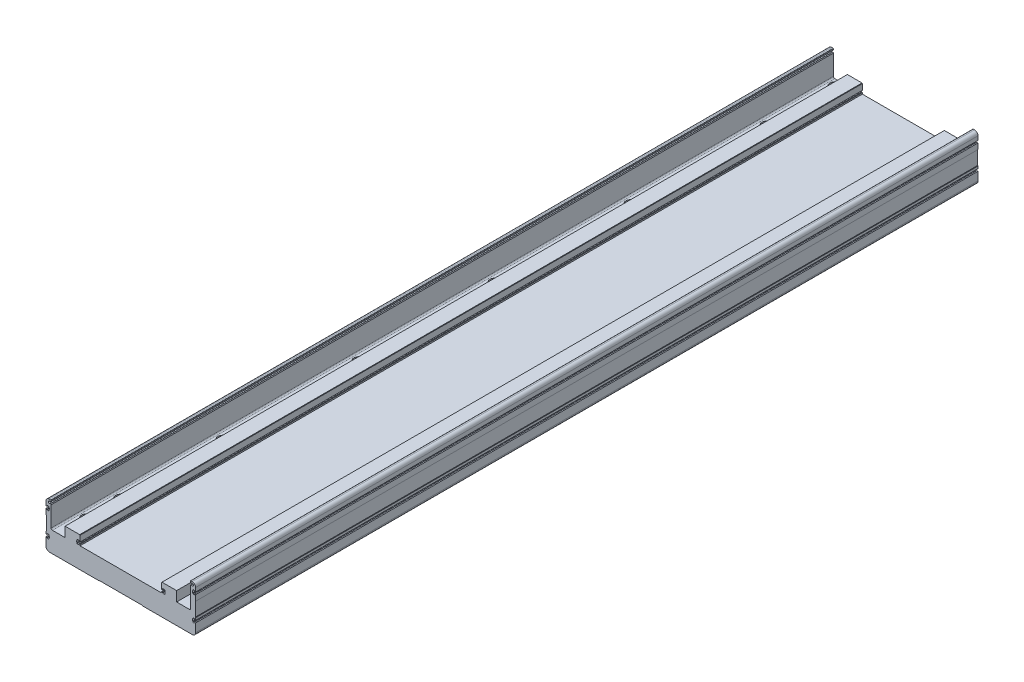
from build123d import *

# Parameters (mm, degrees)
EXTRUDE_1_DEPTH             = 575
FILLET_11_R                 = 2
SKETCH_24_W                 = 220
SKETCH_24_H                 = 1
CUT_EXTRUDE_8_DEPTH         = 1158.277948464
SKETCH_6_W                  = 30
SKETCH_6_H                  = 5
CUT_EXTRUDE_5_DEPTH         = 1158.277948464
HOLE_WIZARD_4_D             = 8.6
HOLE_WIZARD_4_CBORE_D       = 15
HOLE_WIZARD_4_CBORE_DEPTH   = 18
HOLE_WIZARD_4_2_D           = 8.6
HOLE_WIZARD_4_2_CBORE_D     = 15
HOLE_WIZARD_4_2_CBORE_DEPTH = 18
PATTERN_LINEAR_2_COUNT      = 5
PATTERN_LINEAR_2_PITCH      = 200
HOLE_WIZARD_4_3_D           = 8.6
HOLE_WIZARD_4_3_CBORE_D     = 15
HOLE_WIZARD_4_3_CBORE_DEPTH = 18
SKETCH_46_R                 = 3
CUT_EXTRUDE_9_DEPTH         = 8


with BuildPart() as part:
    # 草图1 → 凸台-拉伸1 (new, symmetric)
    with BuildSketch(Plane.XY):
        with BuildLine():
            Line((-104, 0), (-33.5, 0))
            Line((-33.5, 0), (-32, 1.5))
            Line((-32, 1.5), (32, 1.5))
            Line((32, 1.5), (33.5, 0))
            Line((33.5, 0), (104, 0))
            Line((104, 0), (105, 1))
            ThreePointArc((105, 1), (108.535533906, 2.464466094), (110, 6))
            Line((110, 6), (110, 18.35))
            Line((110, 18.35), (108.4, 18.35))
            Line((108.4, 18.35), (108.4, 17.1))
            Line((108.4, 17.1), (105.8, 17.1))
            Line((105.8, 17.1), (105.8, 18.35075775))
            ThreePointArc((105.8, 18.35075775), (105, 20), (105.8, 21.64924225))
            Line((105.8, 21.64924225), (105.8, 22.9))
            Line((105.8, 22.9), (108.4, 22.9))
            Line((108.4, 22.9), (108.4, 21.65))
            Line((108.4, 21.65), (110, 21.65))
            Line((110, 21.65), (110, 25))
            Line((110, 25), (109.5, 25.5))
            Line((109.5, 25.5), (109.5, 45.5))
            Line((109.5, 45.5), (110, 46))
            Line((110, 46), (110, 54.35))
            Line((110, 54.35), (108.4, 54.35))
            Line((108.4, 54.35), (108.4, 53.1))
            Line((108.4, 53.1), (105.8, 53.1))
            Line((105.8, 53.1), (105.8, 54.35075775))
            ThreePointArc((105.8, 54.35075775), (105, 56), (105.8, 57.64924225))
            Line((105.8, 57.64924225), (105.8, 58.9))
            Line((105.8, 58.9), (108.4, 58.9))
            Line((108.4, 58.9), (108.4, 57.65))
            Line((108.4, 57.65), (110, 57.65))
            Line((110, 57.65), (110, 63.5))
            ThreePointArc((110, 63.5), (108.535533906, 67.035533906), (105, 68.5))
            Line((105, 68.5), (103, 68.5))
            ThreePointArc((103, 68.5), (102.646446609, 68.353553391), (102.5, 68))
            Line((102.5, 68), (102.5, 66.45777949))
            Line((102.5, 66.45777949), (103.391660973, 65.566118517))
            ThreePointArc((103.391660973, 65.566118517), (103.542746661, 65.507773508), (103.687494715, 65.580430413))
            ThreePointArc((103.687494715, 65.580430413), (106.7, 64.5), (103.687494715, 63.419569587))
            ThreePointArc((103.687494715, 63.419569587), (103.542746661, 63.492226492), (103.391660973, 63.433881483))
            Line((103.391660973, 63.433881483), (102.5, 62.54222051))
            Line((102.5, 62.54222051), (102.5, 31))
            Line((102.5, 31), (82, 31))
            Line((82, 31), (82, 47))
            Line((82, 47), (62, 47))
            Line((62, 47), (60, 45))
            Line((60, 45), (60, 36.3))
            ThreePointArc((60, 36.3), (60.058578644, 36.158578644), (60.2, 36.1))
            Line((60.2, 36.1), (61, 36.1))
            ThreePointArc((61, 36.1), (61.141421356, 36.158578644), (61.2, 36.3))
            Line((61.2, 36.3), (61.2, 37.8))
            Line((61.2, 37.8), (64.6, 37.8))
            Line((64.6, 37.8), (64.6, 36.132882801))
            ThreePointArc((64.6, 36.132882801), (65, 34.9), (64.6, 33.667117199))
            Line((64.6, 33.667117199), (64.6, 32))
            Line((64.6, 32), (61.2, 32))
            Line((61.2, 32), (61.2, 33.5))
            ThreePointArc((61.2, 33.5), (61.141421356, 33.641421356), (61, 33.7))
            Line((61, 33.7), (60.2, 33.7))
            ThreePointArc((60.2, 33.7), (60.058578644, 33.641421356), (60, 33.5))
            Line((60, 33.5), (60, 31.5))
            Line((60, 31.5), (-60, 31.5))
            Line((-60, 31.5), (-60, 33.5))
            ThreePointArc((-60, 33.5), (-60.058578644, 33.641421356), (-60.2, 33.7))
            Line((-60.2, 33.7), (-61, 33.7))
            ThreePointArc((-61, 33.7), (-61.141421356, 33.641421356), (-61.2, 33.5))
            Line((-61.2, 33.5), (-61.2, 32))
            Line((-61.2, 32), (-64.6, 32))
            Line((-64.6, 32), (-64.6, 33.667117199))
            ThreePointArc((-64.6, 33.667117199), (-65, 34.9), (-64.6, 36.132882801))
            Line((-64.6, 36.132882801), (-64.6, 37.8))
            Line((-64.6, 37.8), (-61.2, 37.8))
            Line((-61.2, 37.8), (-61.2, 36.3))
            ThreePointArc((-61.2, 36.3), (-61.141421356, 36.158578644), (-61, 36.1))
            Line((-61, 36.1), (-60.2, 36.1))
            ThreePointArc((-60.2, 36.1), (-60.058578644, 36.158578644), (-60, 36.3))
            Line((-60, 36.3), (-60, 45))
            Line((-60, 45), (-62, 47))
            Line((-62, 47), (-82, 47))
            Line((-82, 47), (-82, 31))
            Line((-82, 31), (-102.5, 31))
            Line((-102.5, 31), (-102.5, 62.54222051))
            Line((-102.5, 62.54222051), (-103.391660973, 63.433881483))
            ThreePointArc((-103.391660973, 63.433881483), (-103.542746661, 63.492226492), (-103.687494715, 63.419569587))
            ThreePointArc((-103.687494715, 63.419569587), (-106.7, 64.5), (-103.687494715, 65.580430413))
            ThreePointArc((-103.687494715, 65.580430413), (-103.542746661, 65.507773508), (-103.391660973, 65.566118517))
            Line((-103.391660973, 65.566118517), (-102.5, 66.45777949))
            Line((-102.5, 66.45777949), (-102.5, 68))
            ThreePointArc((-102.5, 68), (-102.646446609, 68.353553391), (-103, 68.5))
            Line((-103, 68.5), (-105, 68.5))
            ThreePointArc((-105, 68.5), (-108.535533906, 67.035533906), (-110, 63.5))
            Line((-110, 63.5), (-110, 57.65))
            Line((-110, 57.65), (-108.4, 57.65))
            Line((-108.4, 57.65), (-108.4, 58.9))
            Line((-108.4, 58.9), (-105.8, 58.9))
            Line((-105.8, 58.9), (-105.8, 57.64924225))
            ThreePointArc((-105.8, 57.64924225), (-105, 56), (-105.8, 54.35075775))
            Line((-105.8, 54.35075775), (-105.8, 53.1))
            Line((-105.8, 53.1), (-108.4, 53.1))
            Line((-108.4, 53.1), (-108.4, 54.35))
            Line((-108.4, 54.35), (-110, 54.35))
            Line((-110, 54.35), (-110, 46))
            Line((-110, 46), (-109.5, 45.5))
            Line((-109.5, 45.5), (-109.5, 25.5))
            Line((-109.5, 25.5), (-110, 25))
            Line((-110, 25), (-110, 21.65))
            Line((-110, 21.65), (-108.4, 21.65))
            Line((-108.4, 21.65), (-108.4, 22.9))
            Line((-108.4, 22.9), (-105.8, 22.9))
            Line((-105.8, 22.9), (-105.8, 21.64924225))
            ThreePointArc((-105.8, 21.64924225), (-105, 20), (-105.8, 18.35075775))
            Line((-105.8, 18.35075775), (-105.8, 17.1))
            Line((-105.8, 17.1), (-108.4, 17.1))
            Line((-108.4, 17.1), (-108.4, 18.35))
            Line((-108.4, 18.35), (-110, 18.35))
            Line((-110, 18.35), (-110, 6))
            ThreePointArc((-110, 6), (-108.535533906, 2.464466094), (-105, 1))
            Line((-105, 1), (-104, 0))
        make_face()
    extrude(amount=EXTRUDE_1_DEPTH, both=True)

    # 圆角11
    fillet_11_edges = [part.edges().sort_by_distance(p)[0] for p in [
        (-102.5, 31, 0),
        (102.5, 31, 0),
    ]]
    fillet(fillet_11_edges, radius=FILLET_11_R)

    # 草图24 → 切除-拉伸8 (cut, through all)
    with BuildSketch(Plane.XY.offset(575)):
        with Locations((0, 0.5)):
            Rectangle(SKETCH_24_W, SKETCH_24_H)
    extrude(amount=-CUT_EXTRUDE_8_DEPTH, mode=Mode.SUBTRACT)

    # 草图6 → 切除-拉伸5 (cut, through all)
    with BuildSketch(Plane(origin=(0, 0, -575), x_dir=(-1, 0, 0), z_dir=(0, 0, -1))):
        with Locations((-68, 48)):
            Rectangle(SKETCH_6_W, SKETCH_6_H)
        with Locations((68, 48)):
            Rectangle(SKETCH_6_W, SKETCH_6_H)
    extrude(amount=-CUT_EXTRUDE_5_DEPTH, mode=Mode.SUBTRACT)

    # Hole Wizard 4 (through all)
    with Locations(Plane(origin=(268.504354656, 31, 525.723917262), x_dir=(1, 0, 0), z_dir=(0, 1, 0))):
        with Locations((-359.504354656, 991.723917262), (-177.504354656, 991.723917262)):
            hole_wizard_4 = CounterBoreHole(HOLE_WIZARD_4_D / 2, HOLE_WIZARD_4_CBORE_D / 2, HOLE_WIZARD_4_CBORE_DEPTH)

    # Hole Wizard 4 2 (through all)
    with Locations(Plane(origin=(-106.588181769, 31, 143.262217049), x_dir=(1, 0, 0), z_dir=(0, 1, 0))):
        with Locations((197.588181769, -340.737782951), (15.588181769, -340.737782951)):
            CounterBoreHole(HOLE_WIZARD_4_2_D / 2, HOLE_WIZARD_4_2_CBORE_D / 2, HOLE_WIZARD_4_2_CBORE_DEPTH)

    # 阵列(线性)2: Hole Wizard 4 ×5
    with Locations(*[(0, 0, i * PATTERN_LINEAR_2_PITCH) for i in range(1, PATTERN_LINEAR_2_COUNT)]):
        add(hole_wizard_4, mode=Mode.SUBTRACT)

    # Hole Wizard 4 3 (through all)
    with Locations(Plane(origin=(87.957598752, 31, 219.296413073), x_dir=(1, 0, 0), z_dir=(0, 1, 0))):
        with Locations((3.042401248, 785.296413073), (-178.957598752, 785.296413073), (-178.957598752, -314.703586927), (3.042401248, -314.703586927)):
            CounterBoreHole(HOLE_WIZARD_4_3_D / 2, HOLE_WIZARD_4_3_CBORE_D / 2, HOLE_WIZARD_4_3_CBORE_DEPTH)

    # 草图46 → 切除-拉伸9 (cut)
    with BuildSketch(Plane.XZ.offset(-1.5)):
        with Locations(Location((0, -566, 0), (0, 0, 270))):
            Circle(SKETCH_46_R)
        with Locations(Location((0, 484, 0), (0, 0, 270))):
            Circle(SKETCH_46_R)
        with BuildLine():
            Line((3, -515), (3, -517))
            ThreePointArc((3, -517), (0, -520), (-3, -517))
            Line((-3, -517), (-3, -515))
            ThreePointArc((-3, -515), (0, -512), (3, -515))
        make_face()
        with BuildLine():
            Line((-3, 533), (-3, 535))
            ThreePointArc((-3, 535), (0, 538), (3, 535))
            Line((3, 535), (3, 533))
            ThreePointArc((3, 533), (0, 530), (-3, 533))
        make_face()
    extrude(amount=-CUT_EXTRUDE_9_DEPTH, mode=Mode.SUBTRACT)


solid = part.part
